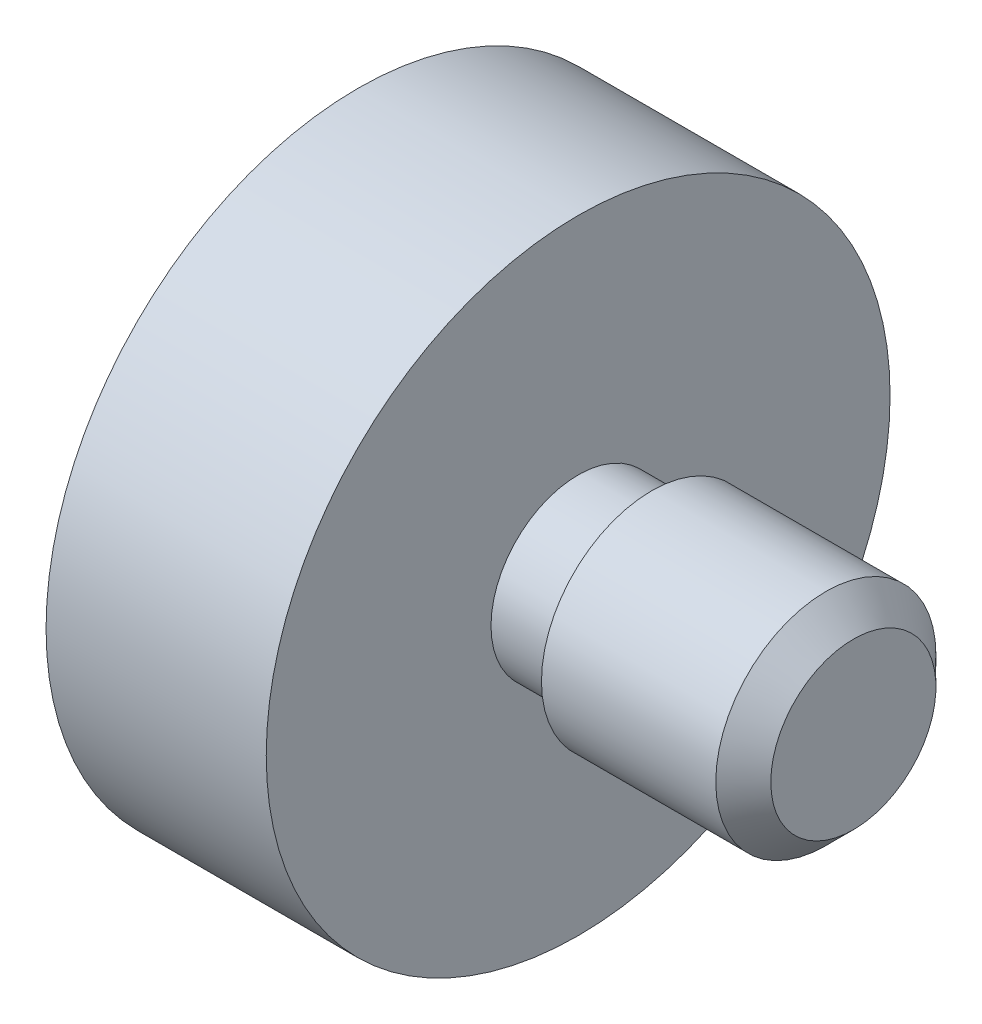
SolidWorks part; units mm, degrees
ref_plane "Front Plane" through (0, 0, 0) normal (0, 0, 1) x (1, 0, 0)
ref_plane "Top Plane" through (0, 0, 0) normal (0, 1, 0) x (1, 0, 0)
ref_plane "Right Plane" through (0, 0, 0) normal (1, 0, 0) x (0, 0, -1)
sketch "Sketch1" plane through (0, 0, 0) normal (0, 0, 1) x (1, 0, 0)
  line L0 (0, 0) -> (35.4304, 0) construction
  line L1 (0, 0) -> (0, 17)
  line L2 (0, 17) -> (12, 17)
  line L3 (12, 17) -> (12, 4.75)
  line L4 (12, 4.75) -> (16, 4.75)
  line L5 (16, 4.75) -> (16, 6)
  line L6 (16, 6) -> (27, 6)
  line L7 (27, 6) -> (27, 0)
  line L8 (0, 0) -> (27, 0)
  dimension "D1" = 4
  dimension "D2" = 15
  dimension "D3" = 27
  dimension "D4" = 6
  dimension "D5" = 17
  dimension "D6" = 4.75
revolve "Revolve1" add sketch "Sketch1" angle 360 about L0
chamfer "Chamfer1" distance 1.5 angle 45 1 edges at (27, 0, 6)
sketch "Sketch2" plane through (0, 0, 0) normal (0, 0, 1) x (1, 0, 0)
  line L0 (-2.4669, 11) -> (8.1777, 11) construction
  line L1 (0, 11) -> (0, 13)
  line L2 (0, 17) -> (0, -17) construction
  line L3 (0, 13) -> (6, 13)
  line L4 (6, 13) -> (7.1547, 11)
  line L5 (0, 11) -> (7.1547, 11)
  dimension "D1" = 11
  dimension "D2" = 2
  dimension "D3" = 60
  dimension "D4" = 6
revolve "Cut-Revolve1" cut sketch "Sketch2" angle 360 about L0
mirror "Mirror1" about plane through (0, 0, 0) normal (0, 1, 0) of "Cut-Revolve1"
